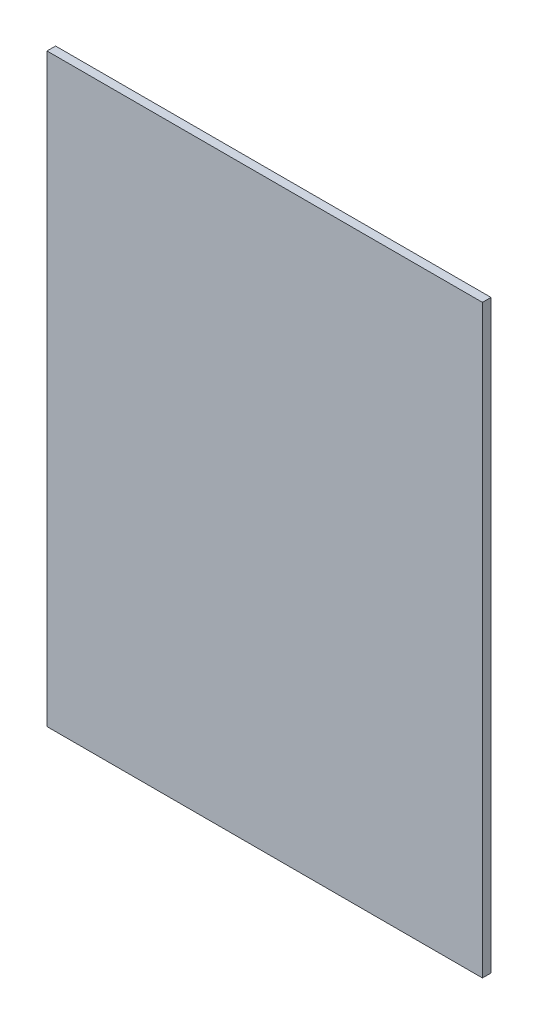
from build123d import *

# Parameters (mm, degrees)
SKETCH1_W      = 101.6
SKETCH1_H      = 136.525
EXTRUDE1_DEPTH = 2


with BuildPart() as part:
    # Sketch1 → Extrude1 (new body)
    with BuildSketch(Plane.XY):
        with Locations((50.8, 68.2625)):
            Rectangle(SKETCH1_W, SKETCH1_H)
    extrude(amount=EXTRUDE1_DEPTH)


solid = part.part
